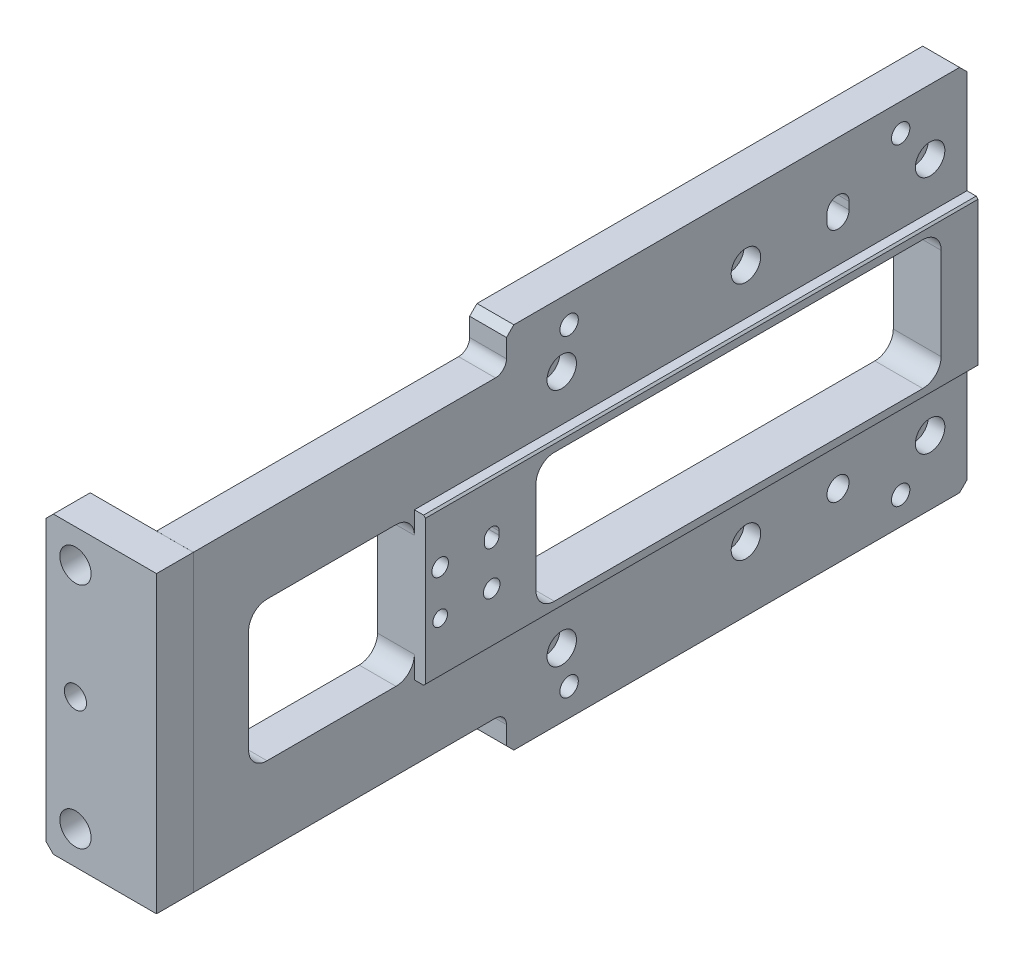
SolidWorks part; units mm, degrees
ref_plane "Front Plane" through (0, 0, 0) normal (0, 0, 1) x (1, 0, 0)
ref_plane "Top Plane" through (0, 0, 0) normal (0, 1, 0) x (1, 0, 0)
ref_plane "Right Plane" through (0, 0, 0) normal (1, 0, 0) x (0, 0, -1)
sketch "Sketch1" plane through (0, 0, 0) normal (0, 1, 0) x (1, 0, 0)
  line L1 (0, 0) -> (20, 0)
  line L2 (0, 0) -> (0, 220)
  line L3 (0, 220) -> (10, 220)
  line L4 (20, 0) -> (20, 8)
  line L7 (20, 8) -> (10, 8)
  line L8 (10, 220) -> (10, 8)
  dimension "D1" = 8
  dimension "D2" = 10
  dimension "D3" = 220
  dimension "D4" = 20
extrude "Boss-Extrude1" add sketch "Sketch1" along normal blind 80
chamfer "Chamfer1" distance 10 angle 45 2 edges at (20, 80, -4) (20, 0, -4)
sketch "Sketch2" plane through (0, 0, 0) normal (0, -1, 0) x (1, 0, 0)
  line L0 (10, -8) -> (10, -220) construction
  line L1 (10, -10) -> (-20, -10)
  line L2 (10, -10) -> (10, 0)
  line L3 (10, 0) -> (-20, 0)
  line L4 (-20, -10) -> (-20, 0)
  line L5 (0, 0) -> (10, 0) construction
  dimension "D1" = 30
  dimension "D2" = 10
extrude "Boss-Extrude2" add sketch "Sketch2" against normal up to surface (80 mm away) up to face at (6, 80, -89.6)
sketch "Sketch3" plane through (0, 0, 0) normal (0, -1, 0) x (1, 0, 0)
  line L1 (10, -8) -> (20, -8)
  line L2 (10, -8) -> (10, 0)
  line L3 (10, 0) -> (20, 0)
  line L4 (20, -8) -> (20, 0)
extrude "Cut-Extrude1" cut sketch "Sketch3" against normal blind 96
sketch "Sketch4" plane through (10, 0, 0) normal (1, 0, 0) x (0, 0, -1)
  line L0 (0, 40) -> (50000, 40) construction
  line L1 (0, 80) -> (0, 0) construction
  line L2 (220, 80) -> (220, 0) construction
  line L3 (70, 60) -> (220, 60)
  line L5 (70, 20) -> (220, 20)
  line L6 (220, 60) -> (220, 20)
  line L7 (70, 60) -> (70, 20)
  point P4 (0, 40)
  dimension "D1" = 40
  dimension "D2" = 150
extrude "Boss-Extrude3" add sketch "Sketch4" along normal blind 3
sketch "Sketch5" plane through (0, 0, 0) normal (0, 0, -1) x (-1, 0, 0)
  line L0 (-11, 40) -> (49989, 40) construction
  line L1 (-13, 20) -> (-13, 60) construction
  line L3 (20, 80) -> (20, 0) construction
  circle A0 centre (12, 71) radius 4.25
  circle A1 centre (12, 9) radius 4.25
  point P4 (-13, 40)
  dimension "D1" = 62
  dimension "D3" = 8.5
  dimension "D2" = 8
extrude "Cut-Extrude2" cut sketch "Sketch5" along normal up to next
chamfer "Chamfer5" distance 0.5 angle 45 2 edges at (13, 60, -145) (13, 20, -145)
sketch "Sketch13" plane through (13, 0, 0) normal (1, 0, 0) x (0, 0, -1)
  line L0 (165, 40) -> (-49835, 40) construction
  line L1 (220, 20.5) -> (220, 59.5) construction
  line L2 (210, 72.5) -> (-49790, 72.5) construction
  circle A0 centre (210, 72.5) radius 2.25
  circle A1 centre (110, 72.5) radius 2.25
  circle A2 centre (210, 7.5) radius 2.25
  circle A3 centre (110, 7.5) radius 2.25
  circle A4 centre (160, 72.5) radius 2.25
  circle A5 centre (160, 7.5) radius 2.25
  point P4 (220, 40)
  dimension "D1" = 4.5
  dimension "D2" = 10
  dimension "D3" = 100
  dimension "D4" = 65
  dimension "D5" = 50
  dimension "D6" = 4.5
extrude "Cut-Extrude7" cut sketch "Sketch13" against normal blind 150
sketch "Sketch14" plane through (13, 0, 0) normal (1, 0, 0) x (0, 0, -1)
  circle A0 centre (110, 72.5) radius 4
  circle A1 centre (110, 7.5) radius 4
  circle A2 centre (210, 7.5) radius 4
  circle A3 centre (210, 72.5) radius 4
  circle A4 centre (160, 72.5) radius 4
  circle A5 centre (160, 7.5) radius 4
  dimension "D1" = 8
extrude "Cut-Extrude8" cut sketch "Sketch14" against normal blind 7.5
sketch "Sketch15" plane through (0, 0, 0) normal (-1, 0, 0) x (0, 0, 1)
  line L0 (-220, 40) -> (49780, 40) construction
  line L2 (-220, -10) -> (-95, -10)
  line L3 (-220, 80) -> (-95, 80)
  line L4 (-220, 80) -> (-220, 90)
  line L5 (-220, 90) -> (-95, 90)
  line L6 (-95, 80) -> (-95, 90)
  line L7 (-95, 0) -> (-95, -10)
  line L8 (-220, 0) -> (-95, 0)
  line L9 (-220, 0) -> (-220, -10)
  line L10 (-220, 80) -> (-220, 0) construction
  line L11 (-220, 0) -> (-10, 0) construction
  point P16 (-220, 40)
  dimension "D1" = 100
  dimension "D2" = 125
extrude "Boss-Extrude5" add sketch "Sketch15" against normal up to surface (10 mm away) up to face at (10, 7.5, -156)
sketch "Sketch9" plane through (10, 0, 0) normal (1, 0, 0) x (0, 0, -1)
  line L0 (142.9464, 82.5) -> (-49857.0536, 82.5) construction
  line L1 (202, 70) -> (202, -49930) construction
  line L2 (0, 40) -> (50000, 40) construction
  line L3 (0, 80) -> (0, 0) construction
  line L4 (220, 90) -> (220, 60) construction
  circle A0 centre (202, 82.5) radius 1
  circle A1 centre (112, 82.5) radius 1
  circle A2 centre (112, -2.5) radius 1
  circle A3 centre (202, -2.5) radius 1
  point P12 (0, 40)
  dimension "D1" = 2
  dimension "D2" = 85
  dimension "D3" = 18
  dimension "D4" = 90
extrude "Cut-Extrude4" cut sketch "Sketch9" against normal blind 25
hole_wizard "M6 Tapped Hole1" positions "3DSketch1" profile "Sketch10" tap size "M6" standard "Gb" end condition through all
sketch3d "3DSketch1"
  line L0 (0, 82.5, -202) -> (10, 82.5, -202) construction
  line L1 (0, 82.5, -112) -> (10, 82.5, -112) construction
  line L2 (0, -2.5, -112) -> (10, -2.5, -112) construction
  line L3 (0, -2.5, -202) -> (10, -2.5, -202) construction
  point P0 (10, 82.5, -202)
  point P4 (10, 82.5, -112)
  point P8 (10, -2.5, -112)
  point P12 (10, -2.5, -202)
cosmetic thread "Cosmetic thread 1" parameters "D2"=6
cosmetic thread "Cosmetic thread 2" parameters "D2"=6
cosmetic thread "Cosmetic thread 3" parameters "D2"=6
cosmetic thread "Cosmetic thread 4" parameters "D2"=6
sketch "Sketch10" plane through (10, 82.5, -202) normal (0, 1, 0) x (0, 0, -1)
  line L0 (0, 0) -> (0, 30)
  line L1 (0, 30) -> (2.5, 30)
  line L2 (2.5, 30) -> (2.5, 0)
  line L5 (2.5, 0) -> (0, 0)
  line L11 (0, -6.35) -> (0, 107.95) construction
  dimension "通孔螺纹孔钻头直径" = 5
  dimension "通孔螺纹孔钻头深度" = 30
sketch "Sketch18" plane through (10, 0, 0) normal (1, 0, 0) x (0, 0, -1)
  line L0 (0, 40) -> (50000, 40) construction
  line L1 (0, 80) -> (0, 0) construction
  line L3 (25, 59) -> (70, 59)
  line L5 (25, 21) -> (70, 21)
  line L6 (70, 59) -> (70, 21)
  line L9 (25, 21) -> (25, 59)
  point P4 (0, 40)
  dimension "D1" = 38
  dimension "D2" = 70
  dimension "D3" = 25
extrude "Cut-Extrude10" cut sketch "Sketch18" against normal blind 10
fillet "Fillet2" radius 5 4 edges at (5, 21, -70) (5, 59, -70) (5, 59, -25) (5, 21, -25)
fillet "Fillet3" radius 3 2 edges
chamfer "Chamfer6" distance 2 angle 45 6 edges at (5, 90, -220) (5, -10, -220) (5, 90, -95) (5, -10, -95) (-20, 80, -5) (-20, 0, -5)
hole_wizard "Hole size per socket head cap screw type 5" positions "Sketch20" profile "Sketch19" counterbore size "M4" standard "Gb" end condition through all
sketch "Sketch20" plane through (0, 0, 0) normal (-1, 0, 0) x (0, 0, 1)
  line L0 (-70, 26) -> (-70, 54) construction
  line L1 (-65, 59) -> (-30, 59) construction
  point P0 (-88, 34)
  point P3 (-74, 46)
  dimension "D1" = 14
  dimension "D2" = 4
  dimension "D3" = 12
  dimension "D4" = 13
sketch "Sketch19" plane through (0, 34, -88) normal (0, 1, 0) x (0, 0, 1)
  line L0 (0, 0) -> (0, 13)
  line L1 (0, 13) -> (2.25, 13)
  line L3 (2.25, 13) -> (2.25, 5)
  line L4 (2.25, 5) -> (3.75, 5)
  line L5 (3.75, 5) -> (3.75, 0)
  line L7 (3.75, 0) -> (0, 0)
  line L11 (0, -6.35) -> (0, 107.95) construction
  dimension "通孔孔直径" = 4.5
  dimension "通孔孔深度" = 13
  dimension "柱形沉头孔直径" = 7.5
  dimension "柱形沉头孔深度" = 5
hole_wizard "Ø4.0 (4) Diameter Hole1" positions "Sketch22" profile "Sketch21" hole size "Ø4.0" standard "Gb" end condition through all
sketch "Sketch22" plane through (0, 0, 0) normal (-1, 0, 0) x (0, 0, 1)
  line L1 (-70, 26) -> (-70, 54) construction
  line L2 (-65, 59) -> (-30, 59) construction
  point P0 (-74, 34)
  point P3 (-88, 46)
  dimension "D1" = 14
  dimension "D2" = 4
  dimension "D3" = 12
  dimension "D4" = 13
sketch "Sketch21" plane through (0, 34, -74) normal (0, 1, 0) x (0, 0, 1)
  line L0 (0, 0) -> (0, 13)
  line L1 (0, 13) -> (2, 13)
  line L2 (2, 13) -> (2, 0)
  line L5 (2, 0) -> (0, 0)
  line L11 (0, -6.35) -> (0, 107.95) construction
  dimension "通孔孔直径" = 4
  dimension "通孔孔深度" = 13
sketch "Sketch23" plane through (13, 0, 0) normal (1, 0, 0) x (0, 0, -1)
  line L0 (220, 40) -> (0, 40) construction
  line L1 (105, 57.5) -> (205, 57.5)
  line L2 (100, 52.5) -> (100, 27.5)
  line L3 (105, 22.5) -> (205, 22.5)
  line L4 (210, 52.5) -> (210, 27.5)
  line L5 (100, 57.5) -> (210, 22.5) construction
  line L6 (100, 22.5) -> (210, 57.5) construction
  line L7 (220, 20.5) -> (220, 59.5) construction
  line L8 (0, 80) -> (0, 0) construction
  arc A0 (100, 27.5) -> (105, 22.5) centre (105, 27.5) ccw
  arc A1 (205, 22.5) -> (210, 27.5) centre (205, 27.5) ccw
  arc A2 (210, 52.5) -> (205, 57.5) centre (205, 52.5) ccw
  arc A3 (105, 57.5) -> (100, 52.5) centre (105, 52.5) ccw
  point P0 (155, 40)
  dimension "D4" = 5
  dimension "D1" = 110
  dimension "D2" = 10
  dimension "D3" = 35
extrude "Cut-Extrude11" cut sketch "Sketch23" against normal through all
sketch "Sketch24" plane through (0, 0, 0) normal (-1, 0, 0) x (0, 0, 1)
  line L0 (-185, 71.5) -> (-185, 73.5) construction
  line L1 (-188, 71.5) -> (-188, 73.5)
  line L2 (-182, 71.5) -> (-182, 73.5)
  line L3 (-220, 40) -> (0, 40) construction
  line L4 (-220, 88) -> (-220, -8) construction
  line L6 (0, 78) -> (0, 2) construction
  circle A0 centre (-185, 7.5) radius 3
  arc A1 (-188, 71.5) -> (-182, 71.5) centre (-185, 71.5) ccw
  arc A2 (-182, 73.5) -> (-188, 73.5) centre (-185, 73.5) ccw
  point P4 (-185, 72.5)
  dimension "D1" = 6
  dimension "D2" = 6
  dimension "D3" = 2
  dimension "D4" = 65
  dimension "D5" = 35
extrude "Cut-Extrude12" cut sketch "Sketch24" against normal through all
sketch "Sketch25" plane through (0, 0, 0) normal (0, -1, 0) x (1, 0, 0)
  line L0 (0, -92) -> (0, -10) construction
  line L1 (0, -10) -> (10, -10)
  line L2 (0, -10) -> (0, -10.01)
  line L3 (0, -10.01) -> (10, -10.01)
  line L4 (10, -10) -> (10, -10.01)
  line L5 (10, 0) -> (10, -92) construction
  line L6 (-18, -10) -> (0, -10) construction
  dimension "D1" = 0.01
extrude "Cut-Extrude13" cut sketch "Sketch25" against normal through all
sketch "Sketch26" plane through (0, 0, -10) normal (0, 0, -1) x (-1, 0, 0)
  line L0 (-13, 40) -> (20, 40) construction
  line L1 (-13, 20.5) -> (-13, 59.5) construction
  line L2 (20, 78) -> (20, 2) construction
  circle A0 centre (12, 40) radius 3
  dimension "D2" = 6
  dimension "D1" = 8
extrude "Cut-Extrude14" cut sketch "Sketch26" against normal through all
sketch "Sketch28" plane through (0, 0, 0) normal (-1, 0, 0) x (0, 0, 1)
  line L0 (-88, 46.5) -> (-88, 45.5) construction
  line L1 (-86, 46.5) -> (-86, 45.5)
  line L2 (-90, 46.5) -> (-90, 45.5)
  arc A0 (-86, 46.5) -> (-90, 46.5) centre (-88, 46.5) ccw
  arc A1 (-90, 45.5) -> (-86, 45.5) centre (-88, 45.5) ccw
  point P2 (-88, 46)
  dimension "D1" = 4
  dimension "D2" = 1
extrude "Cut-Extrude15" cut sketch "Sketch28" against normal through all
